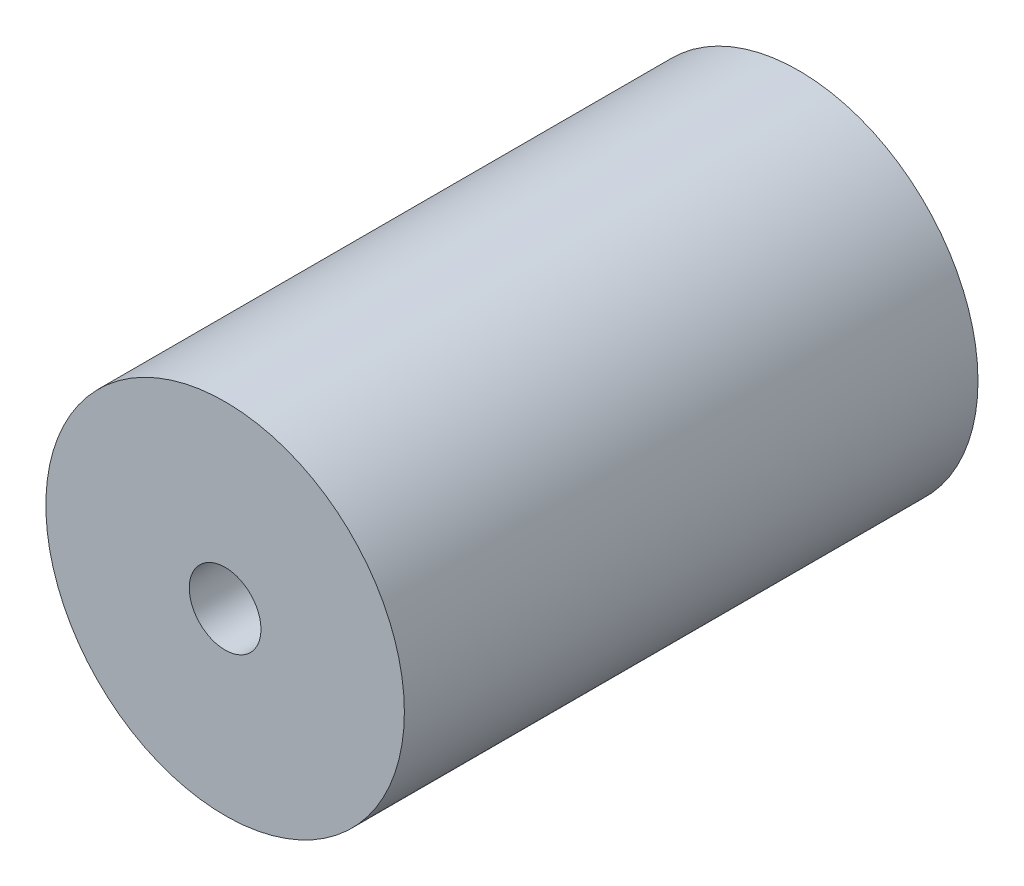
SolidWorks part; units mm, degrees
ref_plane "Front Plane" through (0, 0, 0) normal (0, 0, 1) x (1, 0, 0)
ref_plane "Top Plane" through (0, 0, 0) normal (0, 1, 0) x (1, 0, 0)
ref_plane "Right Plane" through (0, 0, 0) normal (1, 0, 0) x (0, 0, -1)
sketch "Sketch1" plane through (0, 0, 0) normal (0, 0, 1) x (1, 0, 0)
  circle A0 centre (0, 0) radius 25
  circle A1 centre (0, 0) radius 5
  dimension "D1" = 50
  dimension "D2" = 10
extrude "Boss-Extrude1" add sketch "Sketch1" along normal blind 80
